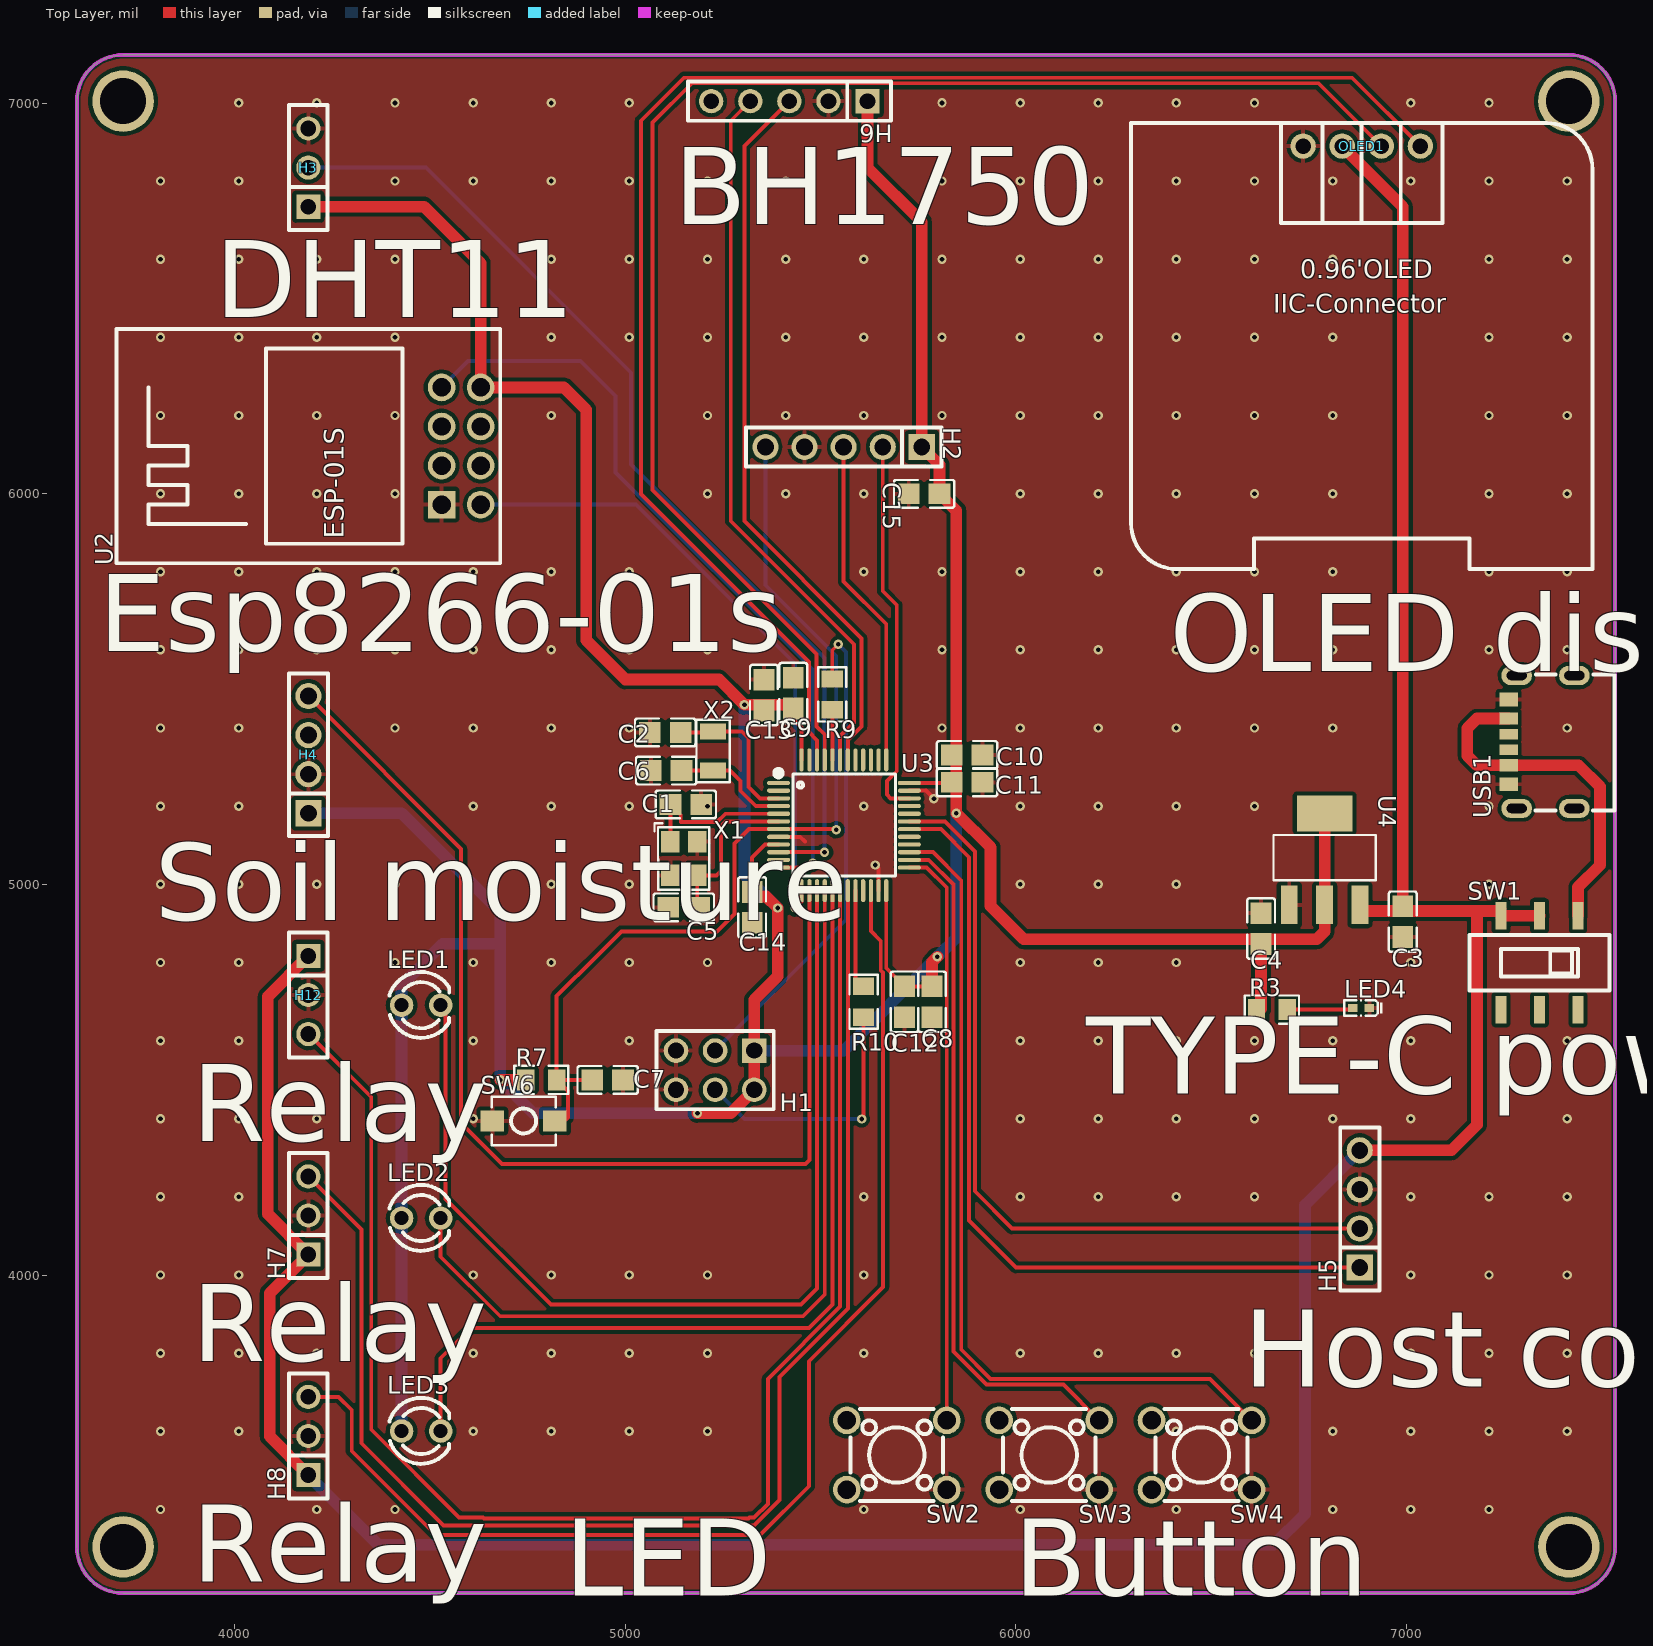
[diagram p0: Top Layer view]
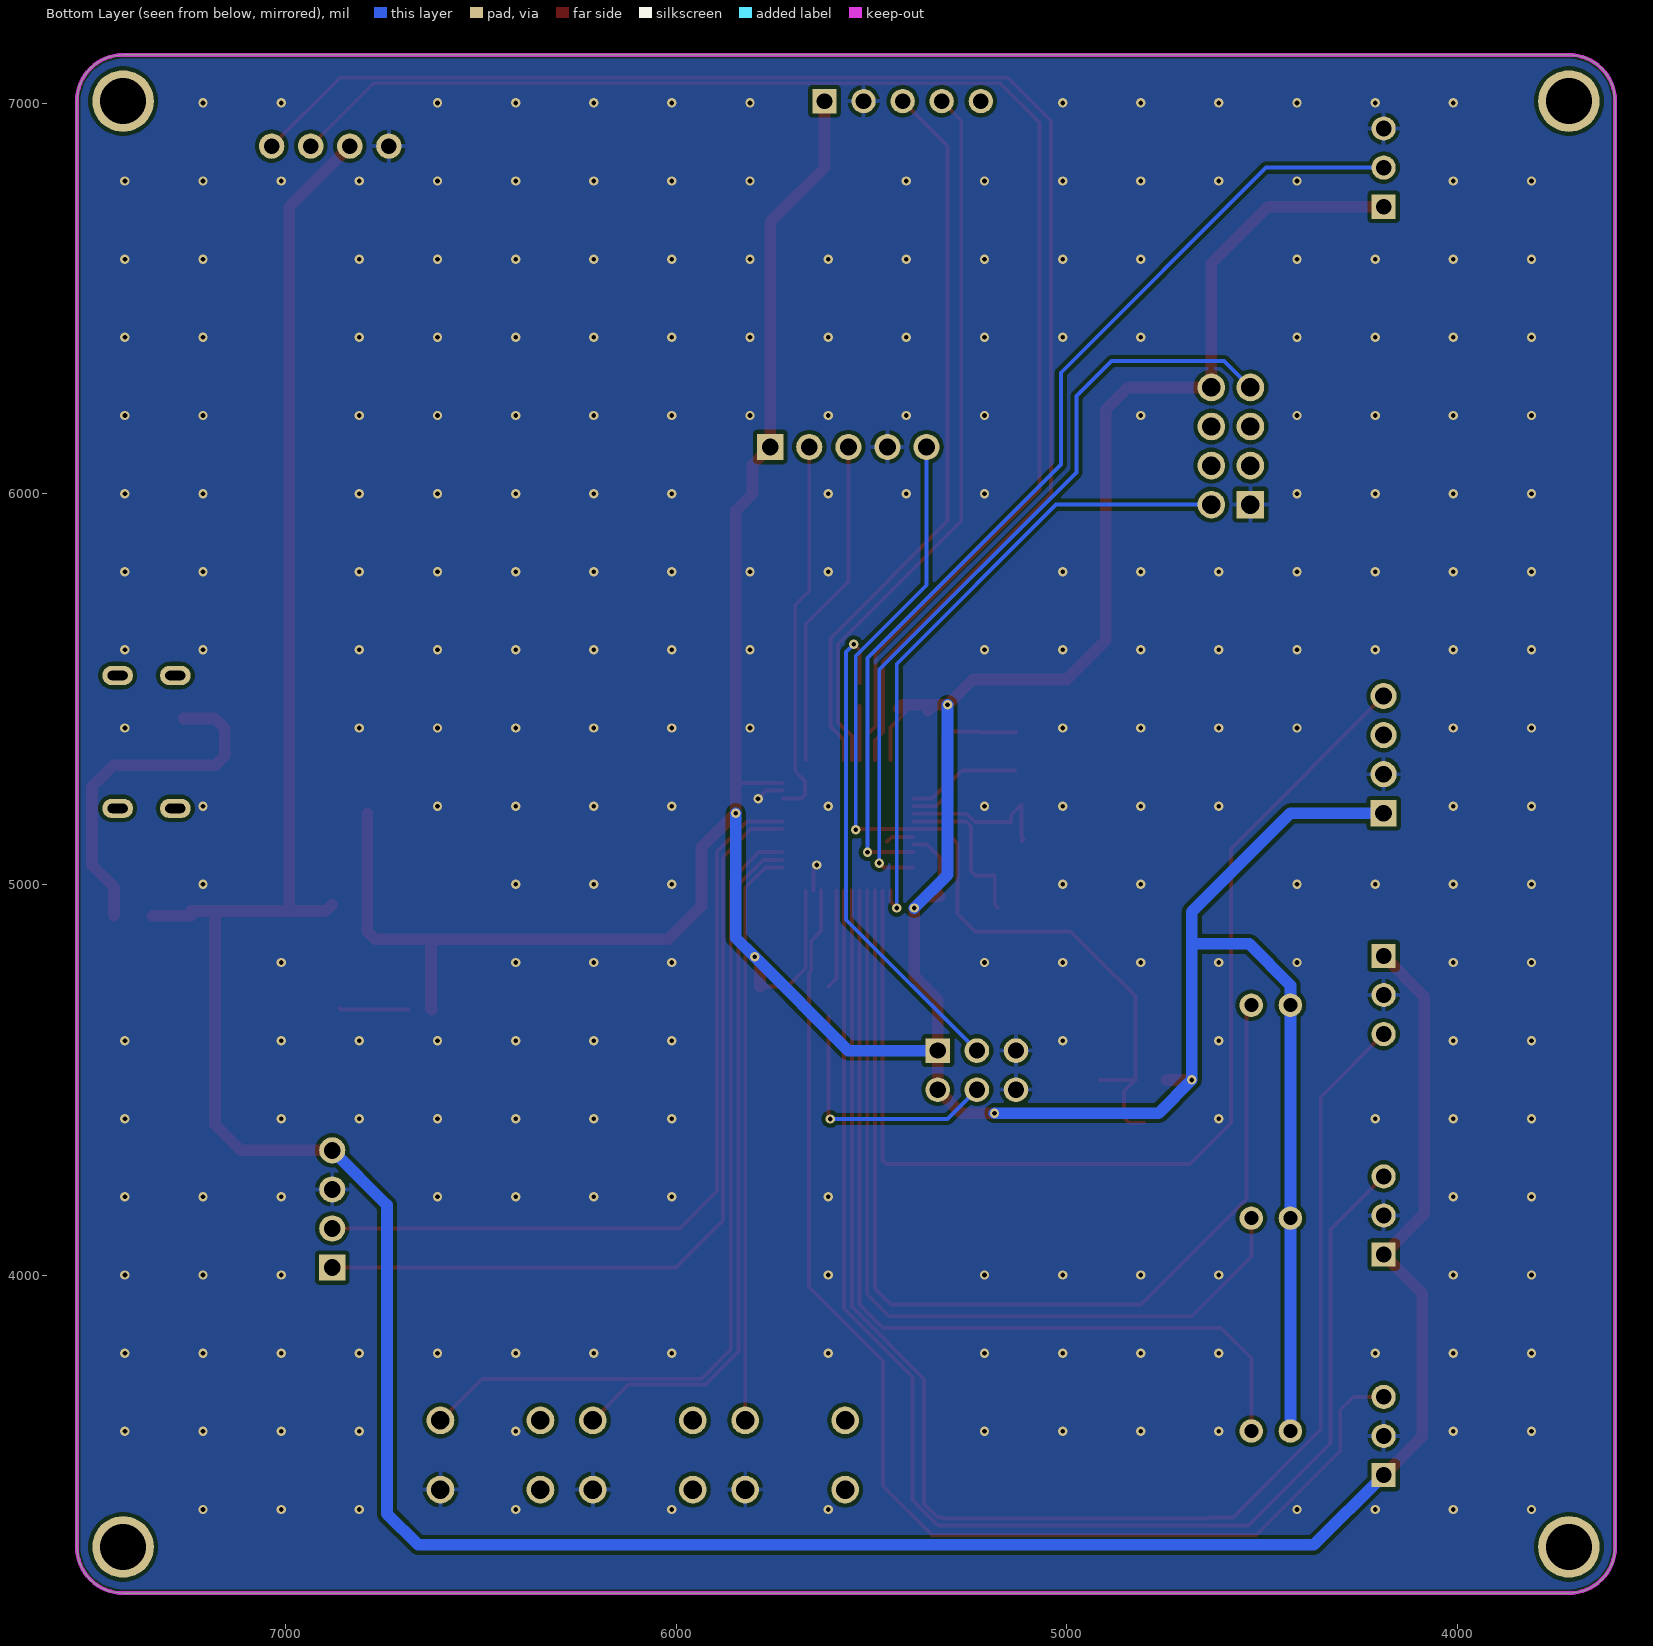
[diagram p1: Bottom Layer view, seen from below]
# Altium PCB MISC62726.pcbdoc
Units mil, origin at the board's own origin, x right, y up, seen from the top; angles counter-clockwise.
Board outline 3937.01 x 3937.01 mil, 2 copper layers (Top Layer, Bottom Layer), stack 62.206 mil thick; 44 components, 47 nets, 186 pads, 265 vias.

## Layer stack, top to bottom
Top Solder Mask Layer: solder mask 0.394, Dk 3.3
Top Layer: signal copper 1.379
Dielectric1: surface 59.449, FR4, Dk 4.5
Bottom Layer: signal copper 1.378
Bottom Solder Mask Layer: solder mask 0.394, Dk 3.3

## Board outline
3714.61,7123.5 ccw(c3714.61,7005.39) 3596.5,7005.39 3596.5,3304.61 ccw(c3714.61,3304.61) 3714.61,3186.5 7415.39,3186.5 ccw(c7415.39,3304.61) 7533.5,3304.61 7533.5,7005.39 ccw(c7415.39,7005.39) 7415.39,7123.5 3714.61,7123.5

## Design rules (kind name [scope] priority, off if disabled: settings)
BoardOutlineClearance copperThickness2oz_1 [All] p2 off: genericclearance=7.99 ignorepadtopadclearanceinfootprint=FALSE except(0: Arc-SplitContinuation Track-SplitContinuation SMDPad-SplitContinuation THPad-SplitContinuation Via-SplitContinuation Fill-SplitContinuation Region-SplitContinuation Poly-SplitContinuation Text-SplitContinuation Hole-SplitContinuation; 5.98: Arc-CutoutEdge Track-CutoutEdge SMDPad-CutoutEdge THPad-CutoutEdge Via-CutoutEdge Text-CutoutEdge; 6.9: Hole-OutlineEdge Hole-CutoutEdge; 10: Poly-OutlineEdge Poly-CutoutEdge; 11.81: Arc-OutlineEdge Track-OutlineEdge SMDPad-OutlineEdge THPad-OutlineEdge Via-OutlineEdge Fill-OutlineEdge Region-OutlineEdge Text-OutlineEdge Fill-CutoutEdge Region-CutoutEdge)
BoardOutlineClearance Plane_innerPlane_1 [All] p4 off: genericclearance=4.02 ignorepadtopadclearanceinfootprint=FALSE except(0: Arc-SplitContinuation Track-SplitContinuation SMDPad-SplitContinuation THPad-SplitContinuation Via-SplitContinuation Fill-SplitContinuation Region-SplitContinuation Poly-SplitContinuation Text-SplitContinuation Hole-SplitContinuation; 5.98: Arc-CutoutEdge Track-CutoutEdge SMDPad-CutoutEdge THPad-CutoutEdge Via-CutoutEdge Text-CutoutEdge; 6.9: Hole-OutlineEdge Hole-CutoutEdge; 10: Poly-OutlineEdge Poly-CutoutEdge; 11.81: Arc-OutlineEdge Track-OutlineEdge SMDPad-OutlineEdge THPad-OutlineEdge Via-OutlineEdge Fill-OutlineEdge Region-OutlineEdge Text-OutlineEdge Fill-CutoutEdge Region-CutoutEdge)
BoardOutlineClearance Copper_copperRegion_1 [All] p6 off: genericclearance=4.02 ignorepadtopadclearanceinfootprint=FALSE except(0: Arc-SplitContinuation Track-SplitContinuation SMDPad-SplitContinuation THPad-SplitContinuation Via-SplitContinuation Fill-SplitContinuation Region-SplitContinuation Poly-SplitContinuation Text-SplitContinuation Hole-SplitContinuation; 5.98: Arc-CutoutEdge Track-CutoutEdge SMDPad-CutoutEdge THPad-CutoutEdge Via-CutoutEdge Text-CutoutEdge; 6.9: Hole-OutlineEdge Hole-CutoutEdge; 10: Poly-OutlineEdge Poly-CutoutEdge; 11.81: Arc-OutlineEdge Track-OutlineEdge SMDPad-OutlineEdge THPad-OutlineEdge Via-OutlineEdge Fill-OutlineEdge Region-OutlineEdge Text-OutlineEdge Fill-CutoutEdge Region-CutoutEdge)
BoardOutlineClearance Copper_copperRegion_copperThickness1oz_1 [All] p8 off: genericclearance=4.02 ignorepadtopadclearanceinfootprint=FALSE except(0: Arc-SplitContinuation Track-SplitContinuation SMDPad-SplitContinuation THPad-SplitContinuation Via-SplitContinuation Fill-SplitContinuation Region-SplitContinuation Poly-SplitContinuation Text-SplitContinuation Hole-SplitContinuation; 5.98: Arc-CutoutEdge Track-CutoutEdge SMDPad-CutoutEdge THPad-CutoutEdge Via-CutoutEdge Text-CutoutEdge; 6.9: Hole-OutlineEdge Hole-CutoutEdge; 10: Poly-OutlineEdge Poly-CutoutEdge; 11.81: Arc-OutlineEdge Track-OutlineEdge SMDPad-OutlineEdge THPad-OutlineEdge Via-OutlineEdge Fill-OutlineEdge Region-OutlineEdge Text-OutlineEdge Fill-CutoutEdge Region-CutoutEdge)
BoardOutlineClearance Copper_copperRegion_Copper_copperRegion_1 [All] p10 off: genericclearance=4.02 ignorepadtopadclearanceinfootprint=FALSE except(0: Arc-SplitContinuation Track-SplitContinuation SMDPad-SplitContinuation THPad-SplitContinuation Via-SplitContinuation Fill-SplitContinuation Region-SplitContinuation Poly-SplitContinuation Text-SplitContinuation Hole-SplitContinuation; 5.98: Arc-CutoutEdge Track-CutoutEdge SMDPad-CutoutEdge THPad-CutoutEdge Via-CutoutEdge Text-CutoutEdge; 6.9: Hole-OutlineEdge Hole-CutoutEdge; 10: Poly-OutlineEdge Poly-CutoutEdge; 11.81: Arc-OutlineEdge Track-OutlineEdge SMDPad-OutlineEdge THPad-OutlineEdge Via-OutlineEdge Fill-OutlineEdge Region-OutlineEdge Text-OutlineEdge Fill-CutoutEdge Region-CutoutEdge)
BoardOutlineClearance copperThickness1oz_1 [All] p12: genericclearance=4.02 ignorepadtopadclearanceinfootprint=FALSE except(0: Arc-SplitContinuation Track-SplitContinuation SMDPad-SplitContinuation THPad-SplitContinuation Via-SplitContinuation Fill-SplitContinuation Region-SplitContinuation Poly-SplitContinuation Text-SplitContinuation Hole-SplitContinuation; 5.98: Arc-CutoutEdge Track-CutoutEdge SMDPad-CutoutEdge THPad-CutoutEdge Via-CutoutEdge Text-CutoutEdge; 6.9: Hole-OutlineEdge Hole-CutoutEdge; 10: Poly-OutlineEdge Poly-CutoutEdge; 11.81: Arc-OutlineEdge Track-OutlineEdge SMDPad-OutlineEdge THPad-OutlineEdge Via-OutlineEdge Fill-OutlineEdge Region-OutlineEdge Text-OutlineEdge Fill-CutoutEdge Region-CutoutEdge)
Clearance copperThickness2oz [All] p1 off: gap=7.99 ignorepadtopadclearanceinfootprint=FALSE except(5.98: SMDPad-Track SMDPad-SMDPad THPad-Track SMDPad-THPad THPad-THPad Track-Via SMDPad-Via THPad-Via Via-Via Fill-SMDPad Region-SMDPad Fill-THPad Region-THPad Fill-Via Region-Via Fill-Fill Fill-Region Region-Region Arc-Track Arc-SMDPad Arc-THPad Arc-Via Fill-Arc Region-Arc Arc-Arc Text-Track SMDPad-Text Text-THPad Text-Via Fill-Text Region-Text Arc-Text Text-Text; 6.9: Hole-Track Hole-SMDPad Hole-THPad Hole-Via Fill-Hole Region-Hole Hole-Arc Hole-Text; 10: Poly-Track Poly-SMDPad Poly-THPad Poly-Via Poly-Fill Poly-Region Poly-Poly Poly-Arc Poly-Text Poly-Hole; 11.81: Fill-Track Region-Track)
Clearance Plane_innerPlane [All] p3 off: gap=4.02 ignorepadtopadclearanceinfootprint=FALSE except(5.98: SMDPad-Track SMDPad-SMDPad THPad-Track SMDPad-THPad THPad-THPad Track-Via SMDPad-Via THPad-Via Via-Via Fill-SMDPad Region-SMDPad Fill-THPad Region-THPad Fill-Via Region-Via Fill-Fill Fill-Region Region-Region Arc-Track Arc-SMDPad Arc-THPad Arc-Via Fill-Arc Region-Arc Arc-Arc Text-Track SMDPad-Text Text-THPad Text-Via Fill-Text Region-Text Arc-Text Text-Text; 6.9: Hole-Track Hole-SMDPad Hole-THPad Hole-Via Fill-Hole Region-Hole Hole-Arc Hole-Text; 10: Poly-Track Poly-SMDPad Poly-THPad Poly-Via Poly-Fill Poly-Region Poly-Poly Poly-Arc Poly-Text Poly-Hole; 11.81: Fill-Track Region-Track)
Clearance Copper_copperRegion [All] p5 off: gap=4.02 ignorepadtopadclearanceinfootprint=FALSE except(5.98: SMDPad-Track SMDPad-SMDPad THPad-Track SMDPad-THPad THPad-THPad Track-Via SMDPad-Via THPad-Via Via-Via Fill-SMDPad Region-SMDPad Fill-THPad Region-THPad Fill-Via Region-Via Fill-Fill Fill-Region Region-Region Arc-Track Arc-SMDPad Arc-THPad Arc-Via Fill-Arc Region-Arc Arc-Arc Text-Track SMDPad-Text Text-THPad Text-Via Fill-Text Region-Text Arc-Text Text-Text; 6.9: Hole-Track Hole-SMDPad Hole-THPad Hole-Via Fill-Hole Region-Hole Hole-Arc Hole-Text; 10: Poly-Track Poly-SMDPad Poly-THPad Poly-Via Poly-Fill Poly-Region Poly-Poly Poly-Arc Poly-Text Poly-Hole; 11.81: Fill-Track Region-Track)
Clearance Copper_copperRegion_copperThickness1oz [All] p7 off: gap=4.02 ignorepadtopadclearanceinfootprint=FALSE except(5.98: SMDPad-Track SMDPad-SMDPad THPad-Track SMDPad-THPad THPad-THPad Track-Via SMDPad-Via THPad-Via Via-Via Fill-SMDPad Region-SMDPad Fill-THPad Region-THPad Fill-Via Region-Via Fill-Fill Fill-Region Region-Region Arc-Track Arc-SMDPad Arc-THPad Arc-Via Fill-Arc Region-Arc Arc-Arc Text-Track SMDPad-Text Text-THPad Text-Via Fill-Text Region-Text Arc-Text Text-Text; 6.9: Hole-Track Hole-SMDPad Hole-THPad Hole-Via Fill-Hole Region-Hole Hole-Arc Hole-Text; 10: Poly-Track Poly-SMDPad Poly-THPad Poly-Via Poly-Fill Poly-Region Poly-Poly Poly-Arc Poly-Text Poly-Hole; 11.81: Fill-Track Region-Track)
Clearance Copper_copperRegion_Copper_copperRegion [All] p9 off: gap=4.02 ignorepadtopadclearanceinfootprint=FALSE except(5.98: SMDPad-Track SMDPad-SMDPad THPad-Track SMDPad-THPad THPad-THPad Track-Via SMDPad-Via THPad-Via Via-Via Fill-SMDPad Region-SMDPad Fill-THPad Region-THPad Fill-Via Region-Via Fill-Fill Fill-Region Region-Region Arc-Track Arc-SMDPad Arc-THPad Arc-Via Fill-Arc Region-Arc Arc-Arc Text-Track SMDPad-Text Text-THPad Text-Via Fill-Text Region-Text Arc-Text Text-Text; 6.9: Hole-Track Hole-SMDPad Hole-THPad Hole-Via Fill-Hole Region-Hole Hole-Arc Hole-Text; 10: Poly-Track Poly-SMDPad Poly-THPad Poly-Via Poly-Fill Poly-Region Poly-Poly Poly-Arc Poly-Text Poly-Hole; 11.81: Fill-Track Region-Track)
Clearance copperThickness1oz [All] p11: gap=4.02 ignorepadtopadclearanceinfootprint=FALSE except(5.98: SMDPad-Track SMDPad-SMDPad THPad-Track SMDPad-THPad THPad-THPad Track-Via SMDPad-Via THPad-Via Via-Via Fill-SMDPad Region-SMDPad Fill-THPad Region-THPad Fill-Via Region-Via Fill-Fill Fill-Region Region-Region Arc-Track Arc-SMDPad Arc-THPad Arc-Via Fill-Arc Region-Arc Arc-Arc Text-Track SMDPad-Text Text-THPad Text-Via Fill-Text Region-Text Arc-Text Text-Text; 6.9: Hole-Track Hole-SMDPad Hole-THPad Hole-Via Fill-Hole Region-Hole Hole-Arc Hole-Text; 10: Poly-Track Poly-SMDPad Poly-THPad Poly-Via Poly-Fill Poly-Region Poly-Poly Poly-Arc Poly-Text Poly-Hole; 11.81: Fill-Track Region-Track)
DiffPairsRouting differentialPair [All] p1: maxlimit=6 minlimit=6 mostfreqgap=6 toplayer_minwidth=5 toplayer_prefwidth=10 toplayer_maxwidth=100 toplayer_mingap=6 toplayer_prefgap=6 toplayer_maxgap=6 bottomlayer_minwidth=5 bottomlayer_prefwidth=10 bottomlayer_maxwidth=100 bottomlayer_mingap=6 bottomlayer_prefgap=6 bottomlayer_maxgap=6 maxuncoupledlength=10
HoleToHoleClearance otherClearance [All] p1: gap=11.81 allowstackedmicrovias=TRUE
Length netLength [All] p1: minlimit=0 maxlimit=0
PasteMaskExpansion pasteMaskExpansion [All] p1: expansion=0
PlaneConnect innerPlane [All] p1: planeconnectstyle=Relief reliefexpansion=20 reliefentries=4 reliefconductorwidth=10 reliefairgap=10
PolygonConnect copperRegion_copperThickness1oz [All] p1 off: connectstyle=Relief reliefconductorwidth=10 reliefentries=4 polygonreliefangle="90 Angle" airgapwidth=10 via.connectstyle=Relief via.reliefconductorwidth=10 via.reliefentries=4 via.polygonreliefangle="90 Angle" via.airgapwidth=10
PolygonConnect copperRegion_Copper_copperRegion [All] p2 off: connectstyle=Relief reliefconductorwidth=10 reliefentries=4 polygonreliefangle="90 Angle" airgapwidth=10 via.connectstyle=Relief via.reliefconductorwidth=10 via.reliefentries=4 via.polygonreliefangle="90 Angle" via.airgapwidth=10
PolygonConnect copperRegion [All] p3: connectstyle=Relief reliefconductorwidth=10 reliefentries=4 polygonreliefangle="90 Angle" airgapwidth=10 via.connectstyle=Relief via.reliefconductorwidth=10 via.reliefentries=4 via.polygonreliefangle="90 Angle" via.airgapwidth=10
RoutingVias viaSize [All] p1: holewidth=12.01 width=24.02 viastyle="Through Hole" minholewidth=11.81 minwidth=19.68 maxholewidth=248.03 maxwidth=393.7
SolderMaskExpansion solderMaskExpansion [IsVia] p1: expansion=-1000 istentingtop=TRUE
SolderMaskExpansion solderMaskExpansion [All] p2: expansion=2 istentingtop=FALSE
Width copperThickness2oz_2 [All] p1 off: maxlimit=100 minlimit=8 preferedwidth=10
Width copperThickness1oz_2 [All] p2: maxlimit=100 minlimit=5 preferedwidth=10

## Components (designator, comment, footprint, x,y, rotation, side; value= is the part's Value field where it differs from the comment)
C1 "18pF" C0805 5155,5205 r0 top
C2 "10pF" C0805 5102.34,5389.28 r0 top
C3 "1uF" C0805 6990,4905 r90 top
C4 "1uF" C0805 6627.44,4887.44 r270 top
C5 "18pF" C0805 5149.78,4941.72 r180 top
C6 "10pF" C0805 5104.78,5291.72 r0 top
C7 "1uF" C0805 4955,4500 r0 top
C8 "4.7uF" C0805 5785,4700 r90 top
C9 "100nF" C0805 5430,5490 r90 top
C10 "100nF" C0805 5874.78,5331.72 r0 top
C11 "100nF" C0805 5874.78,5261.72 r180 top
C12 "100nF" C0805 5715,4700 r90 top
C13 "100nF" C0805 5355,5485 r270 top
C14 "100nF" C0805 5324.78,4941.72 r90 top
C15 "100nF" C0805 5765,6000 r0 top
H1 "" HDR-TH_6P-P2.54-V-R2-C3-S2.54_A2541WV-2X3P 5230,4525 r180 top
H2 "PZ254V-11-05P" HDR-TH_5P-P2.54-V-M 5558.98,6119.97 r180 top
H3 "" HDR-TH_3P-P2.54-V-F 4189,6835 r90 top
H4 "" HDR-TH_4P-P2.54-V-F 4189,5332.42 r90 top
H5 "" HDR-TH_4P-P2.54-V-F 6880,4169.8 r90 top
H6 "" HDR-TH_5P-P2.54-V-F 5420,7005 r180 top
H7 "" HDR-TH_3P-P2.54-V-F 4189,4153.01 r90 top
H8 "" HDR-TH_3P-P2.54-V-F 4189,3588.71 r90 top
H12 "" HDR-TH_3P-P2.54-V-F 4189,4717.31 r270 top
LED1 "" LED_TH-3mm 4477.54,4691.28 r0 top
LED2 "" LED_TH-3mm 4477.54,4146.28 r0 top
LED3 "" LED_TH-3mm 4477.54,3601.28 r0 top
LED4 "" LED_0402 6883.17,4684.04 r180 top
OLED1 "" 0.96OLED_4P 6885,6890 r0 top
R3 "1kΩ" R0805 6655,4680 r0 top
R7 "10kΩ" R0805 4785,4500 r180 top
R9 "10kΩ" R0805 5529.78,5486.72 r90 top
R10 "10kΩ" R0805 5610,4700 r90 top
SW1 "SS-3235S-L1" SW-SMD_SS-3235S-LX 7340,4800 r0 top
SW2 "" SW-TH_4P-L6.0-W6.0-P4.50-LS6.5 5695,3540 r180 top
SW3 "" SW-TH_4P-L6.0-W6.0-P4.50-LS6.5 6085,3540 r180 top
SW4 "" SW-TH_4P-L6.0-W6.0-P4.50-LS6.5 6475,3540 r180 top
SW6 "" Key_SMD_3x4x2 4740,4395 r0 top
U2 "ESP-01S" WIFIM-TH_ESP-01S 4580,6122.39 r90 top
U3 "STM32F103C8T6" LQFP-48_L7.0-W7.0-P0.50-LS9.0-BL 5559.78,5151.72 r270 top
U4 "AMS1117-3.3" SOT-223-3_L6.5-W3.4-P2.30-LS7.0-BR 6790,5065 r270 top
USB1 "" "USB_ TYPE-C-6P" 7345,5360 r90 top
X1 "8MHz" OSC-SMD_4P-L3.2-W2.5-BL 5149.78,5066.72 r270 top
X2 "32.768kHz" CRYSTAL-SMD_L3.2-W1.5-1 5224.78,5341.72 r90 top

## Footprints (in the part's own frame and the unit in brackets; to place one, negate y for a bottom-side part, rotate by r counter-clockwise, add the part's x,y. Pads: shape width x height; smd on the part's side, far side on the other; paste and mask are expansions set on the pad)
0.96OLED_4P [mm]
  round 1.65 hole 1 copper offset 0,0: 1(-3.81,-0.001) 2(-1.27,0.002) 3(1.27,0.002) 4(3.81,0.002)
  silkscreen extent -15,-27.5 15,1.5
C0805 [mm]
  rect 1.41x1.35 smd paste-100 mask+0.051: 1(-1,0) 2(1,0)
  silkscreen extent -1.96,-0.9 1.96,0.9
CRYSTAL-SMD_L3.2-W1.5-1 [mm]
  rect 1.05x1.7 smd: 1(-1.275,0) 2(1.275,0)
  silkscreen extent -2.03,-1.08 2.03,1.08
HDR-TH_3P-P2.54-V-F [mil]
  rect 62x62 hole 40.16: 1(-100,0)
  round 62 hole 40.16: 2(0,0) 3(100,0)
  silkscreen extent -160,-49 160,49
HDR-TH_4P-P2.54-V-F [mm]
  rect 1.7x1.7 hole 1.1: 1(-3.81,0)
  round 1.7 hole 1.1: 2(-1.27,0) 3(1.27,0) 4(3.81,0)
  silkscreen extent -5.29,-1.27 5.29,1.27
HDR-TH_5P-P2.54-V-F [mil]
  rect 62x62 hole 40.16: 1(-200,0)
  round 62 hole 40.16: 2(-100,0) 3(0,0) 4(100,0) 5(200,0)
  silkscreen extent -260,-50 260,50
HDR-TH_5P-P2.54-V-M [mm]
  rect 1.7x1.7 hole 1.1: 1(-5.08,0)
  round 1.7 hole 1.1: 2(-2.54,0) 3(0,0) 4(2.54,0) 5(5.08,0)
  silkscreen extent -6.35,-1.27 6.35,1.27
HDR-TH_6P-P2.54-V-R2-C3-S2.54_A2541WV-2X3P [mm]
  rect 1.6x1.6 hole 1.05: 1(-2.54,-1.27)
  round 1.6 hole 1.05: 2(-2.54,1.27) 3(0,-1.27) 4(0,1.27) 5(2.54,-1.27) 6(2.54,1.27)
  silkscreen extent -3.81,-2.54 3.81,2.54
Key_SMD_3x4x2 [mm]
  rect 1.53x1.36 smd paste+0 mask+0.051: 1(-2.035,0) 2(2.035,0)
  silkscreen extent -2.08,-1.58 2.08,1.58
LED_0402 [mil]
  rect 25.1x21.3 smd paste-3937.01 mask+2: 1(-21.2,0) 2(21.2,0)
  silkscreen extent -55,-21 43,21
LED_TH-3mm [mil]
  round 60 hole 36 paste+0 mask+2: 1(-50,0) 2(50,0)
  silkscreen extent -81,-84 72,85
LQFP-48_L7.0-W7.0-P0.50-LS9.0-BL [mm]
  oval 0.27x1.5 smd paste+0 mask+0.05: 1(-2.75,-4.25) 2(-2.25,-4.25) 3(-1.75,-4.25) 4(-1.25,-4.25) 5(-0.75,-4.25) 6(-0.25,-4.25) 7(0.25,-4.25) 8(0.75,-4.25) 9(1.25,-4.25) 10(1.75,-4.25) 11(2.25,-4.25) 12(2.75,-4.25) 25(2.75,4.25) 26(2.25,4.25) 27(1.75,4.25) 28(1.25,4.25) 29(0.75,4.25) 30(0.25,4.25) 31(-0.25,4.25) 32(-0.75,4.25) 33(-1.25,4.25) 34(-1.75,4.25) 35(-2.25,4.25) 36(-2.75,4.25)
  oval 1.5x0.27 smd paste+0 mask+0.05: 13(4.25,-2.75) 14(4.25,-2.25) 15(4.25,-1.75) 16(4.25,-1.25) 17(4.25,-0.75) 18(4.25,-0.25) 19(4.25,0.25) 20(4.25,0.75) 21(4.25,1.25) 22(4.25,1.75) 23(4.25,2.25) 24(4.25,2.75) 37(-4.25,2.75) 38(-4.25,2.25) 39(-4.25,1.75) 40(-4.25,1.25) 41(-4.25,0.75) 42(-4.25,0.25) 43(-4.25,-0.25) 44(-4.25,-0.75) 45(-4.25,-1.25) 46(-4.25,-1.75) 47(-4.25,-2.25) 48(-4.25,-2.75)
  silkscreen extent -3.59,-4.46 3.3,3.34
OSC-SMD_4P-L3.2-W2.5-BL [mm]
  rect 1.4x1.2 smd: 1(-1.1,-0.875) 2(1.1,-0.875) 3(1.1,0.875) 4(-1.1,0.875)
  silkscreen extent -2.29,-1.9 2.03,1.65
R0805 [mm]
  rect 1.133x1.377 smd paste-100 mask+0.051: 1(-1,0) 2(1,0)
  silkscreen extent -1.76,-0.92 1.76,0.92
SOT-223-3_L6.5-W3.4-P2.30-LS7.0-BR [mm]
  rect 2.5x1.1 smd: 1(2.97,-2.3) 2(2.97,0) 3(2.97,2.3)
  rect 2.34x3.6 smd: 4(-2.97,0)
  silkscreen extent -1.57,-3.33 1.37,3.33
SW-SMD_SS-3235S-LX [mm]
  rect 0.7x1.8 smd: 1(-2.5,3.05) 2(0,3.05) 3(2.5,3.05) 4(-2.5,-3.05) 5(0,-3.05) 6(2.5,-3.05)
  silkscreen extent -4.55,-1.8 4.55,1.8
SW-TH_4P-L6.0-W6.0-P4.50-LS6.5 [mm]
  round 1.8 hole 1.2: 1(-3.25,2.25) 2(3.25,2.25) 3(-3.25,-2.25) 4(3.25,-2.25)
  silkscreen extent -3,-3 3,3
"USB_ TYPE-C-6P" [mm]
  oval 1.25x2 hole 0.6 slot 1.3 at 90 deg paste+0 mask+0.05: 7(-4.193,1.611) 8(4.447,1.611) 9(-4.193,-2.139) 10(4.447,-2.139)
  rect 0.7x1.2 smd paste-100 mask+0.05: A5(-0.373,2.139) B5(0.627,2.139)
  rect 0.8x1.2 smd paste-100 mask+0.05: A9(1.647,2.139) B9(-1.393,2.139)
  rect 0.9x1.2 smd paste-100 mask+0.05: A12(2.877,2.139) B12(-2.623,2.139)
  silkscreen extent -4.34,-4.75 4.52,0.39
WIFIM-TH_ESP-01S [mm]
  rect 1.8x1.8 hole 1.2: 1(-3.81,1.27)
  round 1.8 hole 1.2: 2(-1.27,1.27) 3(1.27,1.27) 4(3.81,1.27) 5(3.81,-1.27) 6(1.27,-1.27) 7(-1.27,-1.27) 8(-3.81,-1.27)
  silkscreen extent -7.62,-2.54 7.62,22.4

## Free pads (board coordinates)
  round 157.48 hole 118.11: 1(3714.61,7005.39) 1(3714.61,3304.61) 1(7415.39,7005.39) 1(7415.39,3304.61)

## Via types
v1: diameter 24.02, hole 12, Top Layer to Bottom Layer, 265 vias

## Nets (pads, with @x,y where several pads share a name; then routed paths per layer and width w, separated by ;. In a path a pad name is that pad's centre, name@x,y a point inside that pad or via, vN(x,y) a via of type N, cw(c..) or ccw(c..) an arc to the next point about the centre after c; other vN are vias at no path point)
$1N17200: SW1.3 USB1.A9 USB1.B9 | length 912.6
  Top Layer w30: USB1.A9 7179.84,5424.84 7155,5400 7155,5330 7179.84,5305.16 USB1.B9 7439.84,5305.16 7495,5250 7495,5050 7438.43,4993.43 SW1.3
$1N17257: H1.3 R9.2 | length 1292
  Top Layer w10: R9.2@5529.78,5516.38 5529.78,5599.78 v1(5545,5615)
  Bottom Layer w10: H1.3 5565,4910 5565,5595 v1(5545,5615)
$1N17258: H1.4 R10.1 | length 668.8
  Top Layer w10: v1(5605,4400) 5610,4405 R10.1
  Bottom Layer w10: H1.4 5305,4400 v1(5605,4400)
$1N17275: LED4.2 R3.2 | length 179
  Top Layer w10: R3.2@6684.66,4680 6857.92,4680 LED4.2
+5V: C3.2 H5.4 H7.1 H8.1 H12.1 OLED1.2 SW1.1 SW1.2 U4.3 | length 8507.5
  Top Layer w30: H8.1 4090,3587.71 4090,3954.01 H7.1 4085,4157.01 4085,4713.31 H12.1 ; OLED1.2@6835,6890.05 6990,6735.05 C3.2@6990,4932.56 ; H5.4 7114.8,4319.8 7180,4385 7180,4926.48 7186.08,4932.56 ; U4.3 6896.22,4932.4 6989.84,4932.4 C3.2@6990,4932.56 ; SW1.1 SW1.2 ; SW1.1@7241.57,4932.56 7186.08,4932.56 ; C3.2@6990,4932.56 7186.08,4932.56
  Bottom Layer w30: H8.1 4367.71,3310 6660,3310 6740,3390 6740,4179.8 H5.4
BOOT0: R9.1 U3.44 | length 138.2
  Top Layer w10: R9.1@5529.78,5457.06 5530.25,5456.59 U3.44
BOOT1: R10.2 U3.20 | length 253.6
  Top Layer w10: U3.20 5589.31,4760.06 R10.2
GND: C1.2 C2.1 C3.1 C4.1 C5.2 C6.1 C7.2 C8.1 C9.2 C10.2 C11.1 C12.1 C13.1 C14.1 C15.1 H1.5 H1.6 H2.4 H3.3 H4.2 H5.3 H6.2 H7.2 H8.2 H12.2 LED4.1 OLED1.1 SW2.1 SW3.1 SW4.1 SW6.1 U2.1 U3.8 U3.23 U3.35 U4.1 USB1.A12 USB1.B12 X1.2 X1.4 | length 213
  Top Layer w10: U3.8 5447.81,5122.19 5460,5110 ; v1(5640,5050) 5648.36,5041.64 U3.23 ; U3.35 5769.7,5240.3 v1(5790,5220)
  other v1: 3810.6,3400.6 4010.6,3400.6 4210.6,3400.6 4410.6,3400.6 5610.6,3400.6 6010.6,3400.6 6410.6,3400.6 6810.6,3400.6 7010.6,3400.6 7210.6,3400.6 3810.6,3600.6 4010.6,3600.6 4610.6,3600.6 4810.6,3600.6 5010.6,3600.6 5210.6,3600.6 6410.6,3600.6 6810.6,3600.6 7010.6,3600.6 7210.6,3600.6 7410.6,3600.6 3810.6,3800.6 4010.6,3800.6 4210.6,3800.6 4610.6,3800.6 4810.6,3800.6 5010.6,3800.6 5210.6,3800.6 5610.6,3800.6 6010.6,3800.6 6210.6,3800.6 6410.6,3800.6 6610.6,3800.6 6810.6,3800.6 7010.6,3800.6 7210.6,3800.6 7410.6,3800.6 3810.6,4000.6 4010.6,4000.6 4610.6,4000.6 4810.6,4000.6 5010.6,4000.6 5210.6,4000.6 5610.6,4000.6 7010.6,4000.6 7210.6,4000.6 7410.6,4000.6 3810.6,4200.6 4010.6,4200.6 5610.6,4200.6 6010.6,4200.6 6210.6,4200.6 6410.6,4200.6 6610.6,4200.6 7010.6,4200.6 7210.6,4200.6 7410.6,4200.6 3810.6,4400.6 4010.6,4400.6 4210.6,4400.6 4610.6,4400.6 6010.6,4400.6 6210.6,4400.6 6410.6,4400.6 6610.6,4400.6 6810.6,4400.6 7010.6,4400.6 7410.6,4400.6 3810.6,4600.6 4010.6,4600.6 4610.6,4600.6 5010.6,4600.6 6010.6,4600.6 6210.6,4600.6 6410.6,4600.6 6610.6,4600.6 6810.6,4600.6 7010.6,4600.6 7410.6,4600.6 3810.6,4800.6 4010.6,4800.6 4410.6,4800.6 4610.6,4800.6 4810.6,4800.6 5010.6,4800.6 5210.6,4800.6 6010.6,4800.6 6210.6,4800.6 6410.6,4800.6 7010.6,4800.6 3810.6,5000.6 4010.6,5000.6 4210.6,5000.6 4410.6,5000.6 4810.6,5000.6 5010.6,5000.6 6010.6,5000.6 6210.6,5000.6 6410.6,5000.6 7210.6,5000.6 3810.6,5200.6 4010.6,5200.6 4610.6,5200.6 4810.6,5200.6 5010.6,5200.6 5210.6,5200.6 5610.6,5200.6 6010.6,5200.6 6210.6,5200.6 6410.6,5200.6 6610.6,5200.6 7210.6,5200.6 3810.6,5400.6 4010.6,5400.6 4410.6,5400.6 4610.6,5400.6 4810.6,5400.6 5010.6,5400.6 5810.6,5400.6 6010.6,5400.6 6210.6,5400.6 6410.6,5400.6 6610.6,5400.6 6810.6,5400.6 7410.6,5400.6 3810.6,5600.6 4010.6,5600.6 4210.6,5600.6 4410.6,5600.6 4610.6,5600.6 4810.6,5600.6 5010.6,5600.6 5210.6,5600.6 5810.6,5600.6 6010.6,5600.6 6210.6,5600.6 6410.6,5600.6 6610.6,5600.6 6810.6,5600.6 7210.6,5600.6 7410.6,5600.6 3810.6,5800.6 4010.6,5800.6 4210.6,5800.6 4410.6,5800.6 4610.6,5800.6 4810.6,5800.6 5010.6,5800.6 5610.6,5800.6 5810.6,5800.6 6010.6,5800.6 6210.6,5800.6 6410.6,5800.6 6610.6,5800.6 6810.6,5800.6 7210.6,5800.6 7410.6,5800.6 3810.6,6000.6 4010.6,6000.6 4210.6,6000.6 4410.6,6000.6 5210.6,6000.6 5410.6,6000.6 5610.6,6000.6 6010.6,6000.6 6210.6,6000.6 6410.6,6000.6 6610.6,6000.6 6810.6,6000.6 7210.6,6000.6 7410.6,6000.6 3810.6,6200.6 4010.6,6200.6 4210.6,6200.6 4410.6,6200.6 4810.6,6200.6 5210.6,6200.6 5410.6,6200.6 5610.6,6200.6 5810.6,6200.6 6010.6,6200.6 6210.6,6200.6 6410.6,6200.6 6610.6,6200.6 6810.6,6200.6 7210.6,6200.6 7410.6,6200.6 3810.6,6400.6 4010.6,6400.6 4210.6,6400.6 4410.6,6400.6 4810.6,6400.6 5010.6,6400.6 5210.6,6400.6 5410.6,6400.6 5610.6,6400.6 5810.6,6400.6 6010.6,6400.6 6210.6,6400.6 6410.6,6400.6 6610.6,6400.6 6810.6,6400.6 7210.6,6400.6 7410.6,6400.6 3810.6,6600.6 4010.6,6600.6 4210.6,6600.6 4410.6,6600.6 4810.6,6600.6 5010.6,6600.6 5210.6,6600.6 5410.6,6600.6 5610.6,6600.6 5810.6,6600.6 6010.6,6600.6 6210.6,6600.6 6410.6,6600.6 6610.6,6600.6 6810.6,6600.6 7210.6,6600.6 7410.6,6600.6 3810.6,6800.6 4010.6,6800.6 4410.6,6800.6 4610.6,6800.6 4810.6,6800.6 5010.6,6800.6 5210.6,6800.6 5410.6,6800.6 5810.6,6800.6 6010.6,6800.6 6210.6,6800.6 6410.6,6800.6 6610.6,6800.6 6810.6,6800.6 7010.6,6800.6 7210.6,6800.6 7410.6,6800.6 4010.6,7000.6 4210.6,7000.6 4410.6,7000.6 4610.6,7000.6 4810.6,7000.6 5010.6,7000.6 5810.6,7000.6 6010.6,7000.6 6210.6,7000.6 6410.6,7000.6 6610.6,7000.6 7010.6,7000.6 7210.6,7000.6
NRST: C7.1 H2.5 R7.1 SW6.2 U3.7 | length 2524.3
  Top Layer w10: SW6.2@4802.52,4390.25 4840.25,4390.25 4853.2,4403.2 4853.2,4471.17 R7.1 ; C7.1 R7.1 ; v1(5540,5140) 5538.12,5141.88 U3.7 5316.88,5141.88 5280,5105 5280,4925 5235,4880 4990,4880 4927.44,4817.44 4824.37,4714.37 R7.1
  Bottom Layer w10: H2.5 5358.98,5766.02 5540,5585 v1(5540,5140)
OSC32_IN: C2.2 U3.3 X2.2 | length 407.8
  Top Layer w10: C2.2@5129.9,5389.28 5222.15,5389.28 X2.2 5298.09,5391.91 5315,5375 5315,5250 5344.38,5220.62 U3.3
OSC32_OUT: C6.2 U3.4 X2.1 | length 312.4
  Top Layer w10: C6.2@5132.34,5291.72 5224.59,5291.72 X2.1 5268.48,5291.52 5295,5265 5295,5240 5334.07,5200.93 U3.4
OSC_IN: C1.1 U3.5 X1.1 | length 414.3
  Top Layer w10: X1.1 5110.41,5114.95 5115.63,5120.17 C1.1 5142.13,5178.5 5142.13,5160 5235,5160 5256.25,5181.25 U3.5
OSC_OUT: C5.1 U3.6 X1.3 | length 417.4
  Top Layer w10: C5.1@5177.34,4941.72 5184.23,4948.61 X1.3 5233.41,5023.41 5245,5035 5245,5150 5256.56,5161.56 U3.6
PA0: H3.2 U3.10 | length 2593.2
  Top Layer w10: U3.10 v1(5510,5082.82)
  Bottom Layer w10: H3.2 4490,6835 5015,6310 5015,6075 5510,5580 v1(5510,5082.82)
PA1: U3.11
PA2: U2.4 U3.12 | length 2006.8
  Top Layer w10: U3.12 5468.45,5043.45 v1(5480,5055)
  Bottom Layer w10: U2.4 4597.61,6340 4885,6340 4975,6250 4975,6055 5480,5550 v1(5480,5055)
PA3: U2.8 U3.13 | length 1650
  Top Layer w10: v1(5435,4940) 5451.51,4956.51 U3.13
  Bottom Layer w10: U2.8 5027.61,5972.39 5435,5565 v1(5435,4940)
PA4: H4.4 U3.14 | length 2882.6
  Top Layer w10: H4.4 4580,5091.42 4580,4390 4685,4285 5461.2,4285 5471.2,4295 U3.14
PA5: LED1.2 U3.15 | length 2599.6
  Top Layer w10: LED1.2 4540,4678.82 4540,4195 4810,3925 5450,3925 5490.88,3965.88 U3.15
PA6: LED2.2 U3.16 | length 2201.8
  Top Layer w10: LED2.2 4527.54,4047.46 4680,3895 5455,3895 5510.57,3950.57 U3.16
PA7: LED3.2 U3.17 | length 2305.2
  Top Layer w10: LED3.2 4527.54,3787.54 4605,3865 5470,3865 5530,3925 5530,4984.15 U3.17
PA8: U3.29
PA9: H5.1 U3.30 | length 2162.5
  Top Layer w10: U3.30 5808.12,5141.88 5880,5070 5880,4140 6000.2,4019.8 H5.1
PA10: H5.2 U3.31 | length 2094
  Top Layer w10: U3.31 5818.44,5161.56 5895,5085 5895,4215 5990.2,4119.8 H5.2
PA11: U3.32
PA12: U3.33
PA13: H2.2 U3.34 | length 976.2
  Top Layer w10: H2.2 5658.98,5751.02 5695,5715 5695,5290 5670,5265 5670,5230 5679.38,5220.62 U3.34
PA14: H2.3 U3.37 | length 846.1
  Top Layer w10: H2.3 5558.98,5776.02 5668.05,5666.95 U3.37
PA15: U3.38
PB0: H12.3 U3.18 | length 3849.6
  Top Layer w10: H12.3 4350,4456.31 4350,3605 4575,3380 4635.92,3380 4638.17,3377.75 5315.79,3377.75 5318.04,3380 5330,3380 5365,3415 5365,3735 5549.94,3919.94 U3.18
PB1: H7.3 U3.19 | length 3555.3
  Top Layer w10: H7.3 4325,4117.01 4325,3570 4535,3360 5330,3360 5395,3425 5395,3740 5570,3915 5570,4984.02 U3.19
PB3: U3.39
PB4: U3.40
PB5: U3.41
PB6: H6.3 U3.42 | length 1872.5
  Top Layer w10: H6.3 5305,6890 5305,5930 5605,5630 5605,5405 5569.62,5369.62 U3.42
PB7: H6.4 U3.43 | length 1851.7
  Top Layer w10: H6.4 5270,6955 5270,5930 5585,5615 5585,5415 5549.94,5379.94 U3.43
PB8: OLED1.3 U3.45 | length 3786.9
  Top Layer w10: U3.45 5510.57,5384.43 5490,5405 5490,5590 5070,6010 5070,6950 5170.98,7050.98 6774.07,7050.98 OLED1.3@6935,6890.05
PB9: OLED1.4 U3.46 | length 3935.8
  Top Layer w10: U3.46 5490.88,5369.12 5470,5390 5470,5570 5040,6000 5040,6955 5150,7065 6860.05,7065 OLED1.4@7035,6890.05
PB10: U3.21
PB11: H8.3 U3.22 | length 3156.9
  Top Layer w10: H8.3 4266.29,3688.71 4300,3655 4300,3550 4515,3335 5345,3335 5470,3460 5470,3780 5660,3970 5660,4774.55 5654.03,4780.51 5654.03,4855.97 5628.68,4881.32 U3.22
PB12: SW2.3 U3.25 | length 1480.6
  Top Layer w10: U3.25 5771.55,5043.45 5822.95,4992.05 SW2.3
PB13: SW3.3 U3.26 | length 1780.1
  Top Layer w10: U3.26 5776.86,5063.14 5840,5000 5840,3805 5925,3720 6121.53,3720 SW3.3
PB14: SW4.3 U3.27 | length 2181.2
  Top Layer w10: U3.27 5787.18,5082.82 5860,5010 5860,3810 5935,3735 6496.53,3735 SW4.3
PB15: U3.28
PC13: U3.2
VBAT: U3.1
VCC: C4.2 C8.2 C9.1 C10.1 C11.2 C12.2 C13.2 C14.2 C15.2 H1.1 H1.2 H2.1 H3.1 H4.1 H6.1 LED1.1 LED2.1 LED3.1 R3.1 R7.2 U2.5 U3.9 U3.24 U3.36 U3.48 U4.2 U4.4 | length 12079.8
  Top Layer w10: C14.2@5324.78,4969.28 5324.78,5069.78 5357.51,5102.51 U3.9 ; C9.1@5405.67,5447.35 5451.51,5401.51 U3.48 ; U3.24 5668.05,4786.32 C12.2 C8.2 ; U3.36 5845.49,5259.99 C11.2@5847.22,5261.72
  Top Layer w30: H3.1 4485,6735 4630,6590 U2.5 4842.61,6272.39 4900,6215 4900,5625 5000,5525 5240,5525 v1(5305,5460) C13.2@5340.63,5460 ; v1(4680,4500) R7.2 ; v1(5185,4415) 5270,4415 H1.2 H1.1 5330,4705 5390,4765 v1(5390,4940) 5360.72,4969.28 C14.2@5324.78,4969.28 ; C13.2 C13.2@5340.63,5460 ; C9.1 5420.63,5460 C13.2@5340.63,5460 ; H6.1 5620,6835 5758.98,6696.02 H2.1 5804.37,6074.57 C15.2 5847.22,5957.15 5847.22,5261.72 v1(5847.22,5182.78) 5935,5095 5935,4945 6020.12,4859.88 C4.2@6627.44,4859.88 ; C8.2 5785,4801.07 v1(5798.93,4815) ; R3.1@6625.34,4680 6627.44,4682.1 C4.2@6627.44,4859.88 ; U4.4 U4.2 6790,4880 6769.88,4859.88 C4.2@6627.44,4859.88
  Bottom Layer w30: H4.1 4427.58,5182.42 4680,4930 4680,4848.17 ; LED3.1 LED2.1 LED1.1 4427.54,4742.54 4533.17,4848.17 4680,4848.17 ; v1(5185,4415) 4765,4415 v1(4680,4500) 4680,4848.17 ; v1(5305,5460) 5305,5025 v1(5390,4940) ; H1.1 5558.93,4575 v1(5798.93,4815) 5847.22,4863.29 v1(5847.22,5182.78)
pads on no net: H4.3 H6.5 SW1.4 SW1.5 SW1.6 SW2.2 SW2.4 SW3.2 SW3.4 SW4.2 SW4.4 U2.2 U2.3 U2.6 U2.7 U3.47 USB1.7 USB1.8 USB1.9 USB1.10 USB1.A5 USB1.B5

## Polygon pours and split planes (outlines as drawn)
GND on Bottom Layer (solid, remove dead copper, pour order 2): 3525,7245 3525,3080 7700,3080 7700,7245
GND on Top Layer (solid, remove dead copper, pour order 2): 3000,7415 3000,3000 7930,3000 7930,7415

## Keep-outs
Board Outline Layer:
  the board outline again, w10

## Silkscreen, mask and mechanical layers (free items; w line width, h text height)
Top Silkscreen Layer:
  text "BH1750" at 5125,6690 h196.85
  text "DHT11" at 3950.39,6451.44 h196.85
  text "Esp8266-01s" at 3652.14,5597.68 h196.85
  text "OLED display" at 6393.02,5546.51 h196.85
  text "Soil moisture" at 3795.75,4909.09 h196.85
  text "TYPE-C power interface" at 6180,4465 h196.85
  text "Relay" at 3891.79,4343.6 h196.85
  text "Relay" at 3891.79,3779.3 h196.85
  text "Host computer" at 6583.53,3715 h196.85
  text "Relay" at 3891.79,3215 h196.85
  text "LED" at 4845,3180 h196.85
  text "Button" at 5995,3180 h196.85